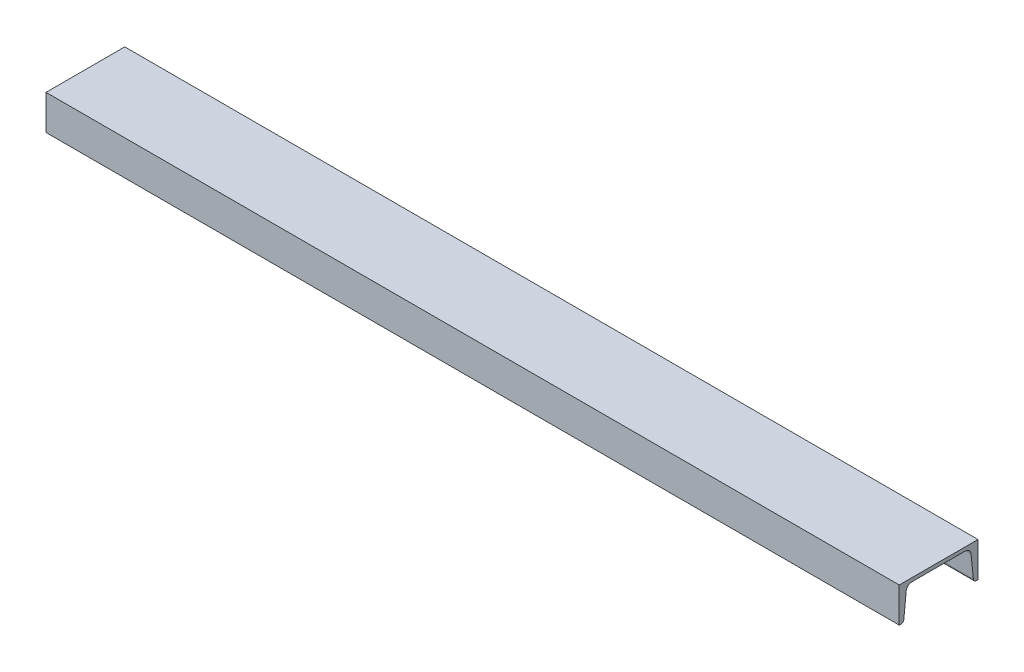
SolidWorks part; units mm, degrees
material "K"
ref_plane "Front" through (0, 0, 0) normal (0, 0, 1) x (1, 0, 0)
ref_plane "Top" through (0, 0, 0) normal (0, 1, 0) x (1, 0, 0)
ref_plane "Right" through (0, 0, 0) normal (1, 0, 0) x (0, 0, -1)
sketch "草图1" plane through (0, 0, 0) normal (0, 0, 1) x (1, 0, 0)
  line L0 (-650, 0) -> (650, 0)
  line L1 (0, 0) -> (0, -328.8235) construction
  dimension "D1" = 1300
other "Structural Member1"
ref_plane "Plane1" through (-650, 0, 0) normal (1, 0, 0) x (0, 1, 0)
sketch "Sketch1" plane through (-650, 0, 0) normal (1, 0, 0) x (0, 1, 0)
  line L0 (0, 0) -> (0, -120)
  line L1 (0, -120) -> (-53, -120)
  line L2 (0, -60) -> (-53, -60) construction
  line L3 (-5.5, -100.4801) -> (-5.5, -19.5199)
  line L4 (-13.6045, -109.4354) -> (-48.9478, -112.9698)
  line L5 (-53, -117.4474) -> (-53, -120)
  line L6 (-53, -120) -> (0, -114.7) construction
  line L7 (-53, -117.4474) -> (-5.5, -117.4474) construction
  line L8 (-53, -2.5526) -> (-53, -117.4474) construction
  line L9 (-53, -2.5526) -> (-53, 0)
  line L10 (0, 0) -> (-53, 0)
  line L11 (-13.6045, -10.5646) -> (-48.9478, -7.0302)
  line L12 (-5.5, -117.4474) -> (-5.5, -100.4801) construction
  line L13 (-29.25, -111) -> (-29.25, -120) construction
  arc A0 (-5.5, -100.4801) -> (-13.6045, -109.4354) centre (-14.5, -100.4801) cw
  arc A1 (-13.6045, -10.5646) -> (-5.5, -19.5199) centre (-14.5, -19.5199) cw
  arc A2 (-48.9478, -112.9698) -> (-53, -117.4474) centre (-48.5, -117.4474) ccw
  arc A3 (-53, -2.5526) -> (-48.9478, -7.0302) centre (-48.5, -2.5526) ccw
  point P2 (-26.5, 0)
  point P5 (-5.5, -60)
  point P10 (-26.5, -120)
  point P20 (-5.5, -11.375)
  point P26 (-53, -6.625)
  point P27 (-29.25, -117.4474)
  point P29 (0, 0)
  dimension "r" = 9
  dimension "r1" = 4.5
  dimension "h" = 120
  dimension "b" = 53
  dimension "d" = 5.5
  dimension "t" = 9
  dimension "a" = 5.3
equation "\"零件重量\"= IIF ( \"SW-质量\" > 100 , int ( \"SW-质量\" ) , \"SW-质量\" )"
